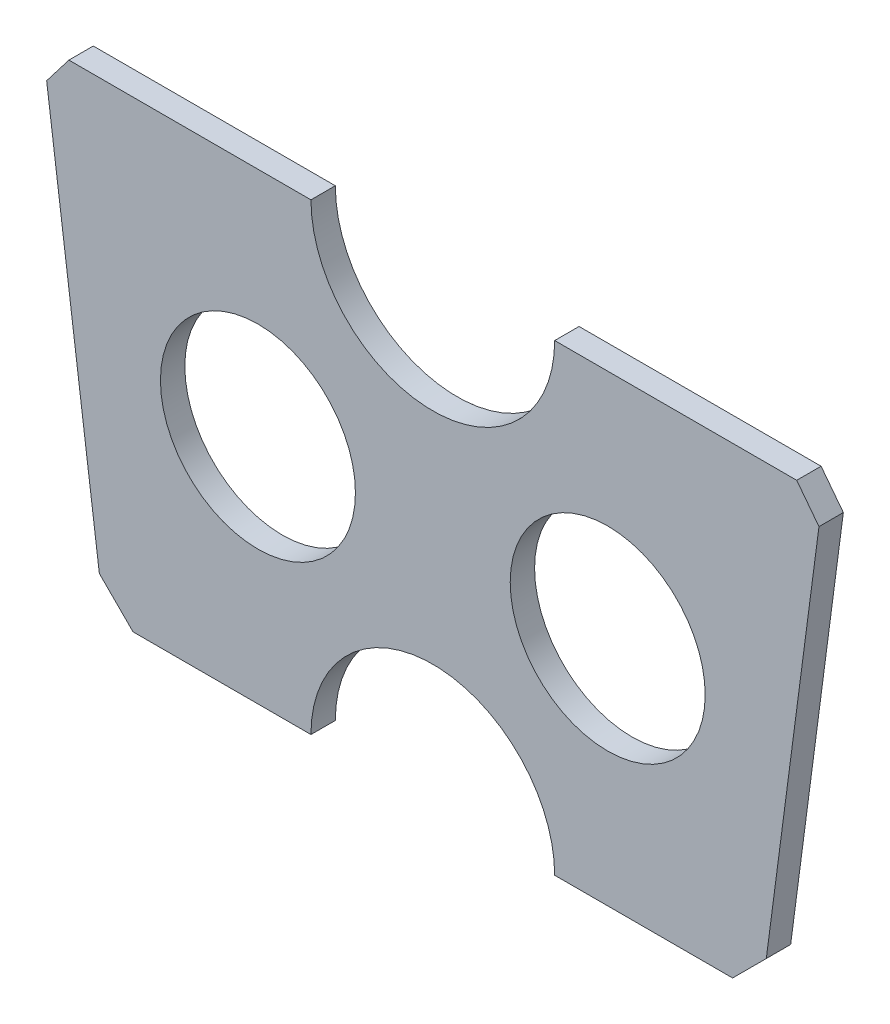
SolidWorks part; units mm, degrees
ref_plane "Front Plane" through (0, 0, 0) normal (0, 0, 1) x (1, 0, 0)
ref_plane "Top Plane" through (0, 0, 0) normal (0, 1, 0) x (1, 0, 0)
ref_plane "Right Plane" through (0, 0, 0) normal (1, 0, 0) x (0, 0, -1)
sketch "Sketch1" plane through (0, 0, 0) normal (0, 0, 1) x (1, 0, 0)
  line L0 (-97.7966, 0) -> (109.1657, 0) construction
  line L1 (50, 95) -> (149.3039, 95)
  line L2 (0, -95) -> (0, 103.4812) construction
  line L3 (71.75, 69.6857) -> (71.75, -26.9526) construction
  line L4 (-50.0516, -95) -> (-50, -95)
  line L5 (158.4345, 83.1025) -> (136.8182, -81.1818)
  line L6 (50, -95) -> (123, -95)
  line L7 (123, -95) -> (136.8182, -81.1818)
  line L8 (149.3039, 95) -> (158.4345, 83.1025)
  line L9 (-50, -95) -> (-123, -95)
  line L10 (-123, -95) -> (-136.8182, -81.1818)
  line L11 (-149.3039, 95) -> (-158.4345, 83.1025)
  line L12 (-158.4345, 83.1025) -> (-136.8182, -81.1818)
  line L13 (-50, 95) -> (-149.3039, 95)
  circle A0 centre (71.75, 0) radius 40
  arc A1 (-50, 95) -> (50, 95) centre (0, 95) ccw
  arc A2 (50, -95) -> (-50, -95) centre (0, -95) ccw
  circle A3 centre (-71.75, 0) radius 40
  point P4 (160, 95)
  point P14 (135, -95)
  point P25 (-135, -95)
  point P28 (-160, 95)
  dimension "D3" = 80
  dimension "D4" = 100
  dimension "D6" = 100
  dimension "D1" = 95
  dimension "D2" = 71.75
  dimension "D5" = 190
  dimension "D7" = 135
  dimension "D8" = 160
  dimension "D9" = 12
  dimension "D10" = 45
  dimension "D11" = 12
  dimension "D12" = 45
extrude "Boss-Extrude1" add sketch "Sketch1" along normal blind 10 contours A2 L6 L7 L5 L8 L1 A1 L13 L11 L12 L10 L9 L4 A0 A3
